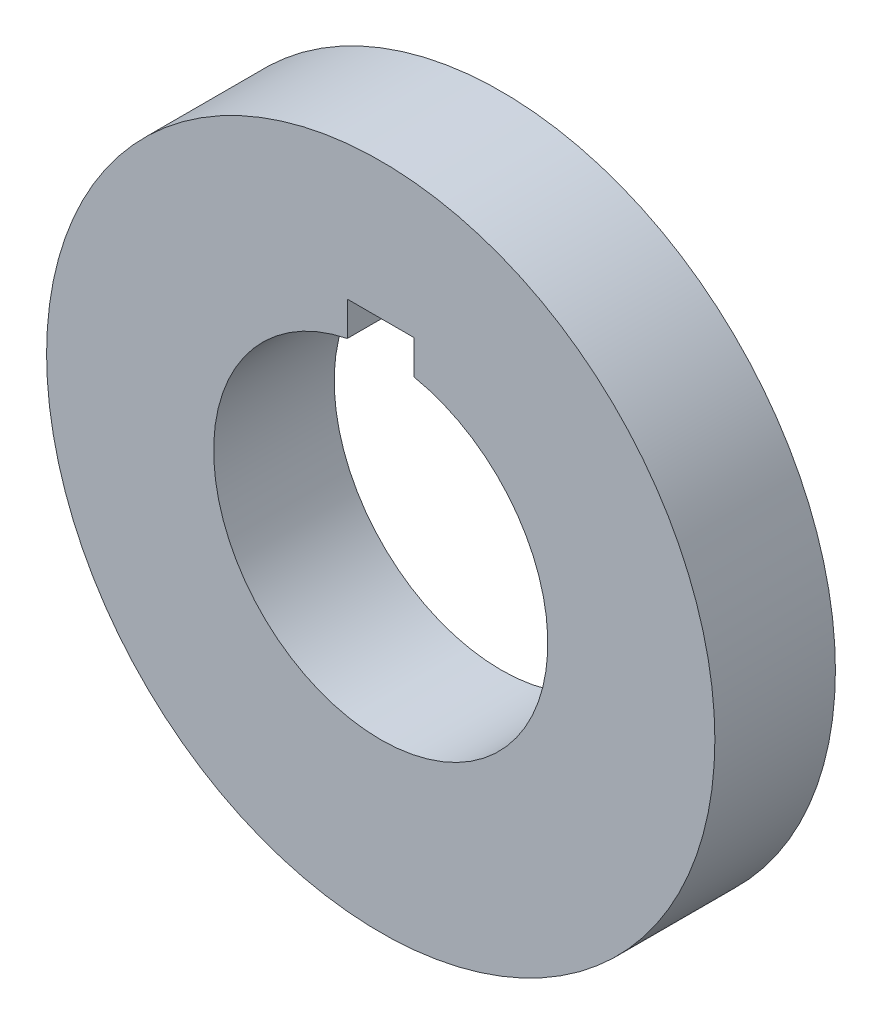
SolidWorks part; units mm, degrees
ref_plane "Front Plane" through (0, 0, 0) normal (0, 0, 1) x (1, 0, 0)
ref_plane "Top Plane" through (0, 0, 0) normal (0, 1, 0) x (1, 0, 0)
ref_plane "Right Plane" through (0, 0, 0) normal (1, 0, 0) x (0, 0, -1)
sketch "Sketch1" plane through (0, 0, 0) normal (0, 0, 1) x (1, 0, 0)
  circle A0 centre (0, 0) radius 25
  circle A1 centre (0, 0) radius 12.5 construction
  circle A2 centre (0, 0) radius 12.5
  dimension "D1" = 50
extrude "Boss-Extrude1" add sketch "Sketch1" against normal blind 17
other "Move Face1" face at (12.5, 0, 0) parameters "D1"=7.9815
sketch "Sketch2" plane through (0, 0, -17) normal (0, 0, -1) x (-1, 0, 0)
  line L1 (-2.5, 10.2) -> (2.5, 10.2)
  line L2 (-2.5, 10.2) -> (-2.5, 14.8)
  line L3 (-2.5, 14.8) -> (2.5, 14.8)
  line L4 (2.5, 10.2) -> (2.5, 14.8)
  line L5 (-2.5, 10.2) -> (2.5, 14.8) construction
  line L6 (-2.5, 14.8) -> (2.5, 10.2) construction
  circle A0 centre (0, 0) radius 12.5 construction
  point P0 (0, 12.5)
  dimension "D1" = 5
  dimension "D2" = 4.6
extrude "Cut-Extrude1" cut sketch "Sketch2" against normal through all
